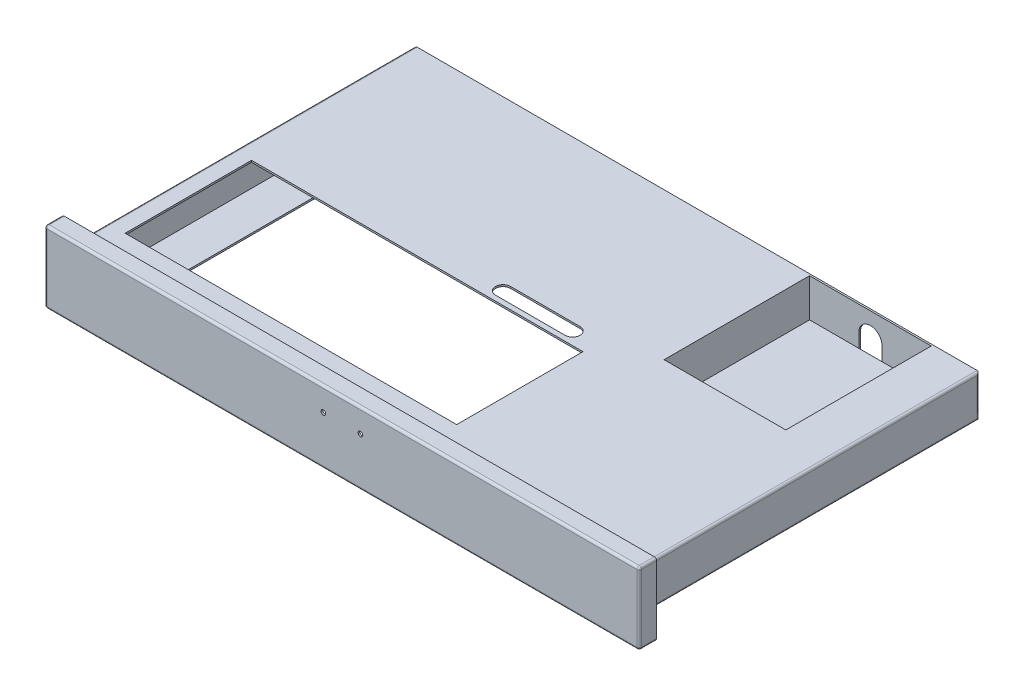
SolidWorks part; units mm, degrees
ref_plane "前视" through (0, 0, 0) normal (0, 0, 1) x (1, 0, 0)
ref_plane "上视" through (0, 0, 0) normal (0, 1, 0) x (1, 0, 0)
ref_plane "右视" through (0, 0, 0) normal (1, 0, 0) x (0, 0, -1)
sketch "草图1" plane through (0, 0, 0) normal (0, 0, 1) x (1, 0, 0)
  line L1 (-256.5, 31) -> (256.5, 31)
  line L2 (-256.5, 31) -> (-256.5, -31)
  line L3 (-256.5, -31) -> (256.5, -31)
  line L4 (256.5, 31) -> (256.5, -31)
  line L5 (-256.5, 31) -> (256.5, -31) construction
  line L6 (-256.5, -31) -> (256.5, 31) construction
  point P0 (0, 0)
  dimension "D1" = 513
  dimension "D2" = 62
extrude "凸台-拉伸1" add sketch "草图1" along normal blind 15
shell "抽壳1" thickness 1.5
sketch "草图2" plane through (0, 0, 0) normal (0, 0, -1) x (-1, 0, 0)
  line L0 (-256.5, -31) -> (-256.5, 31) construction
  line L1 (-243.5, 18) -> (243.5, 18)
  line L2 (-243.5, 18) -> (-243.5, -18)
  line L3 (-243.5, -18) -> (243.5, -18)
  line L4 (243.5, 18) -> (243.5, -18)
  line L5 (-243.5, 18) -> (243.5, -18) construction
  line L6 (-243.5, -18) -> (243.5, 18) construction
  line L7 (-256.5, 31) -> (256.5, 31) construction
  point P0 (0, 0)
  dimension "D1" = 13
  dimension "D2" = 13
extrude "切除-拉伸1" cut sketch "草图2" against normal blind 2
sketch "草图3" plane through (0, 0, 13.5) normal (0, 0, -1) x (-1, 0, 0)
  line L0 (243.5, 18) -> (-243.5, 18) construction
  line L1 (-243.5, 18) -> (-243.5, -18) construction
  line L2 (243.5, -18) -> (243.5, 18) construction
  line L3 (243.5, 18) -> (-243.5, 18)
  line L4 (-243.5, 18) -> (-243.5, -18)
  line L5 (243.5, -18) -> (243.5, 18)
  line L6 (-243.5, -18) -> (-208.5, -18)
  line L7 (-243.5, -18) -> (243.5, -18) construction
  line L8 (243.5, -18) -> (208.5, -18)
  line L9 (242, -16.5) -> (208.5, -16.5)
  line L10 (242, -16.5) -> (242, 16.5)
  line L11 (242, 16.5) -> (-242, 16.5)
  line L12 (-242, 16.5) -> (-242, -16.5)
  line L13 (-242, -16.5) -> (-208.5, -16.5)
  line L14 (-208.5, -18) -> (-208.5, -16.5)
  line L15 (208.5, -18) -> (208.5, -16.5)
  dimension "D1" = 35
  dimension "D2" = 1.5
extrude "凸台-拉伸2" add sketch "草图3" along normal blind 305
sketch "草图4" plane through (0, 0, -291.5) normal (0, 0, -1) x (-1, 0, 0)
  line L0 (-242, 16.5) -> (242, 16.5) construction
  line L1 (-242, -16.5) -> (-242, 16.5) construction
  line L2 (242, 16.5) -> (242, -16.5) construction
  line L3 (-242, 16.5) -> (242, 16.5)
  line L4 (-242, -16.5) -> (-242, 16.5)
  line L5 (242, 16.5) -> (242, -16.5)
  line L6 (242, -16.5) -> (-242, -16.5)
extrude "凸台-拉伸3" add sketch "草图4" against normal blind 1.5
sketch "草图6" plane through (0, 16.5, 0) normal (0, -1, 0) x (1, 0, 0)
  line L0 (-242, -290) -> (242, -290) construction
  line L1 (205, -290) -> (97, -290)
  line L2 (205, -290) -> (205, -163)
  line L3 (205, -163) -> (97, -163)
  line L4 (97, -290) -> (97, -163)
  line L5 (208.5, -291.5) -> (208.5, 0) construction
  dimension "D1" = 108
  dimension "D2" = 127
  dimension "D3" = 3.5
extrude "凸台-拉伸4" add sketch "草图6" along normal up to surface (33 mm away) up to face at (0, -16.5, -290.75)
sketch "草图7" plane through (0, 18, 0) normal (0, 1, 0) x (1, 0, 0)
  line L6 (98.5, 290) -> (203.5, 290)
  line L9 (203.5, 290) -> (203.5, 164.5)
  line L10 (203.5, 164.5) -> (98.5, 164.5)
  line L11 (98.5, 164.5) -> (98.5, 290)
  line L12 (203.5, 290) -> (203.5, 164.5)
  line L13 (203.5, 164.5) -> (98.5, 164.5)
  line L14 (98.5, 164.5) -> (98.5, 290)
  dimension "D1" = 1.5
extrude "切除-拉伸2" cut sketch "草图7" against normal blind 33
sketch "草图8" plane through (0, 0, -291.5) normal (0, 0, -1) x (-1, 0, 0)
  line L0 (-203.5, 1.5) -> (-98.5, 1.5) construction
  line L1 (-203.5, -15) -> (-203.5, 18) construction
  line L2 (-98.5, -15) -> (-98.5, 18) construction
  line L3 (-151, 1.5) -> (-151, 42.2456) construction
  line L4 (-161, -18) -> (-161, -3)
  line L6 (-141, -3) -> (-141, -18)
  line L7 (-141, -18) -> (-161, -18)
  line L8 (-208.5, -18) -> (208.5, -18) construction
  arc A0 (-141, -3) -> (-161, -3) centre (-151, -3) ccw
  dimension "D1" = 20
  dimension "D2" = 15
extrude "切除-拉伸3" cut sketch "草图8" against normal blind 1.5
sketch "草图9" plane through (0, 18, 0) normal (0, 1, 0) x (1, 0, 0)
  line L0 (-243.5, 291.5) -> (-243.5, 0) construction
  line L1 (-228.5, 135.5) -> (57.5, 135.5)
  line L2 (-228.5, 135.5) -> (-228.5, 26.5)
  line L3 (-228.5, 26.5) -> (57.5, 26.5)
  line L4 (57.5, 135.5) -> (57.5, 26.5)
  line L5 (-243.5, 0) -> (243.5, 0) construction
  dimension "D1" = 286
  dimension "D2" = 109
  dimension "D3" = 15
  dimension "D4" = 26.5
extrude "切除-拉伸4" cut sketch "草图9" against normal blind 1.5
sketch "草图10" plane through (0, 18, 0) normal (0, 1, 0) x (1, 0, 0)
  line L0 (-22.5, 146.5) -> (37.5, 146.5) construction
  line L1 (-22.5, 153) -> (37.5, 153)
  line L2 (-22.5, 140) -> (37.5, 140)
  line L3 (57.5, 135.5) -> (-228.5, 135.5) construction
  line L4 (57.5, 26.5) -> (57.5, 135.5) construction
  arc A0 (-22.5, 153) -> (-22.5, 140) centre (-22.5, 146.5) ccw
  arc A1 (37.5, 140) -> (37.5, 153) centre (37.5, 146.5) ccw
  point P2 (7.5, 146.5)
  dimension "D4" = 20
  dimension "D1" = 13
  dimension "D2" = 60
  dimension "D3" = 11
extrude "切除-拉伸5" cut sketch "草图10" against normal blind 10
sketch "草图11" plane through (0, 0, 13.5) normal (0, 0, -1) x (-1, 0, 0)
  line L0 (0, 0) -> (0, 52.2479) construction
  line L1 (-256.5, 31) -> (256.5, 31) construction
  circle A0 centre (-16, 11) radius 2
  circle A1 centre (16, 11) radius 2
  dimension "D2" = 4
  dimension "D1" = 32
  dimension "D3" = 20
extrude "切除-拉伸6" cut sketch "草图11" against normal through all
fillet "圆角1" radius 2 19 edges at (-226, -18, 0) (226, -18, 0) (0, 18, 0) (-243.5, 0, 0) (-243.5, 0, -291.5) (-243.5, 18, -145.75) (-243.5, -18, -145.75) (243.5, 0, 0) (243.5, 0, -291.5) (243.5, -18, -145.75) (243.5, 18, -145.75) (256.5, 0, 15) (0, -31, 15) (0, 31, 15) (-256.5, 0, 15) (256.5, -31, 7.5) (256.5, 31, 7.5) (-256.5, 31, 7.5) (-256.5, -31, 7.5)
